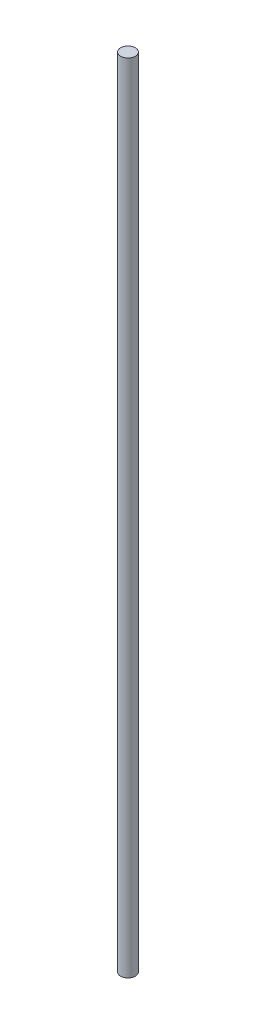
SolidWorks part; units mm, degrees
material "20#"
ref_plane "Front Plane" through (0, 0, 0) normal (0, 0, 1) x (1, 0, 0)
ref_plane "Top Plane" through (0, 0, 0) normal (0, 1, 0) x (1, 0, 0)
ref_plane "Right Plane" through (0, 0, 0) normal (1, 0, 0) x (0, 0, -1)
sketch "Sketch1" plane through (0, 0, 0) normal (0, 1, 0) x (1, 0, 0)
  circle A0 centre (0, 0) radius 1.5
  dimension "D1" = 3
extrude "Boss-Extrude1" add sketch "Sketch1" along normal blind 162
